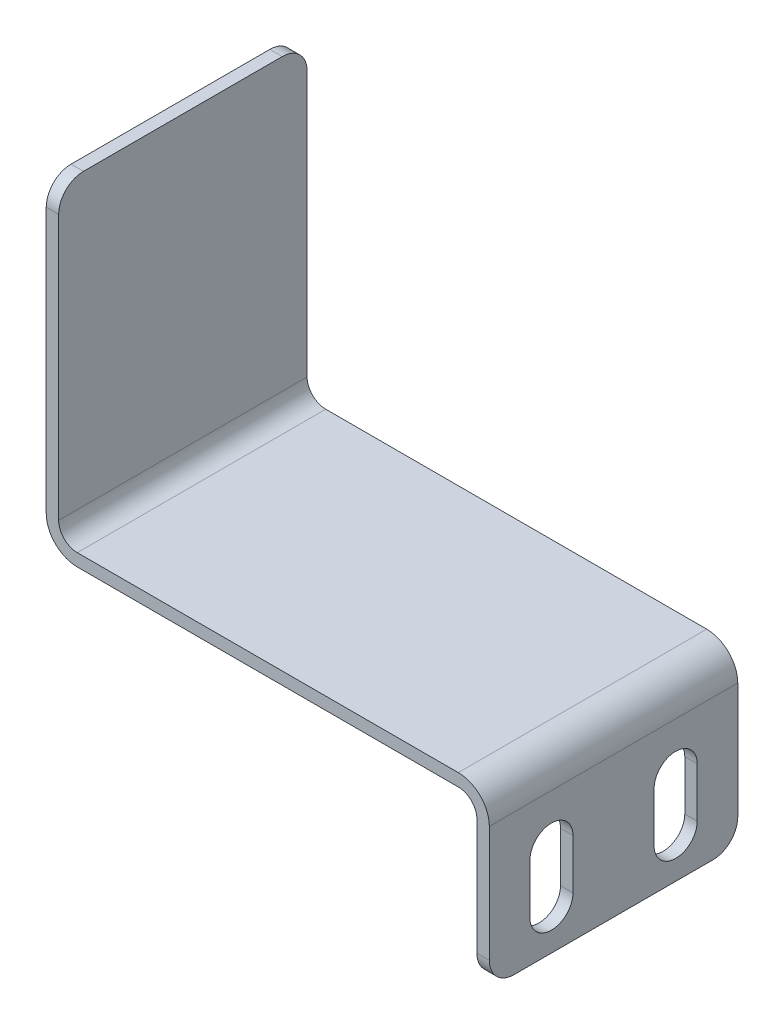
from build123d import *

# Parameters (mm, degrees)
EXTRUDE_1_DEPTH     = 30
FILLET_1_R          = 3
CUT_EXTRUDE_1_DEPTH = 10


with BuildPart() as part:
    # 草图1 → 拉伸-薄壁1 (new body)
    with BuildSketch(Plane.XY):
        with BuildLine():
            Line((0.75, 0), (0.75, 17))
            ThreePointArc((0.75, 17), (-0.348349571, 19.651650429), (-3, 20.75))
            Line((-3, 20.75), (-49, 20.75))
            ThreePointArc((-49, 20.75), (-50.590990258, 21.409009742), (-51.25, 23))
            Line((-51.25, 23), (-51.25, 58))
            Line((-51.25, 58), (-52.75, 58))
            Line((-52.75, 58), (-52.75, 23))
            ThreePointArc((-52.75, 23), (-51.651650429, 20.348349571), (-49, 19.25))
            Line((-49, 19.25), (-3, 19.25))
            ThreePointArc((-3, 19.25), (-1.409009742, 18.590990258), (-0.75, 17))
            Line((-0.75, 17), (-0.75, 0))
            Line((-0.75, 0), (0.75, 0))
        make_face()
    extrude(amount=EXTRUDE_1_DEPTH)

    # 圆角1
    fillet_1_edges = [part.edges().sort_by_distance(p)[0] for p in [
        (0, 0, 0),
        (-52, 58, 0),
        (0, 0, 30),
        (-52, 58, 30),
    ]]
    fillet(fillet_1_edges, radius=FILLET_1_R)

    # 草图2 → 切除-拉伸1 (cut)
    with BuildSketch(Plane.ZY.offset(0.75)):
        with BuildLine():
            Line((10.1, 11), (10.1, 5))
            ThreePointArc((10.1, 5), (7.5, 2.4), (4.9, 5))
            Line((4.9, 5), (4.9, 11))
            ThreePointArc((4.9, 11), (7.5, 13.6), (10.1, 11))
        make_face()
        with BuildLine():
            Line((25.1, 11), (25.1, 5))
            ThreePointArc((25.1, 5), (22.5, 2.4), (19.9, 5))
            Line((19.9, 5), (19.9, 11))
            ThreePointArc((19.9, 11), (22.5, 13.6), (25.1, 11))
        make_face()
    extrude(amount=-CUT_EXTRUDE_1_DEPTH, mode=Mode.SUBTRACT)


solid = part.part
